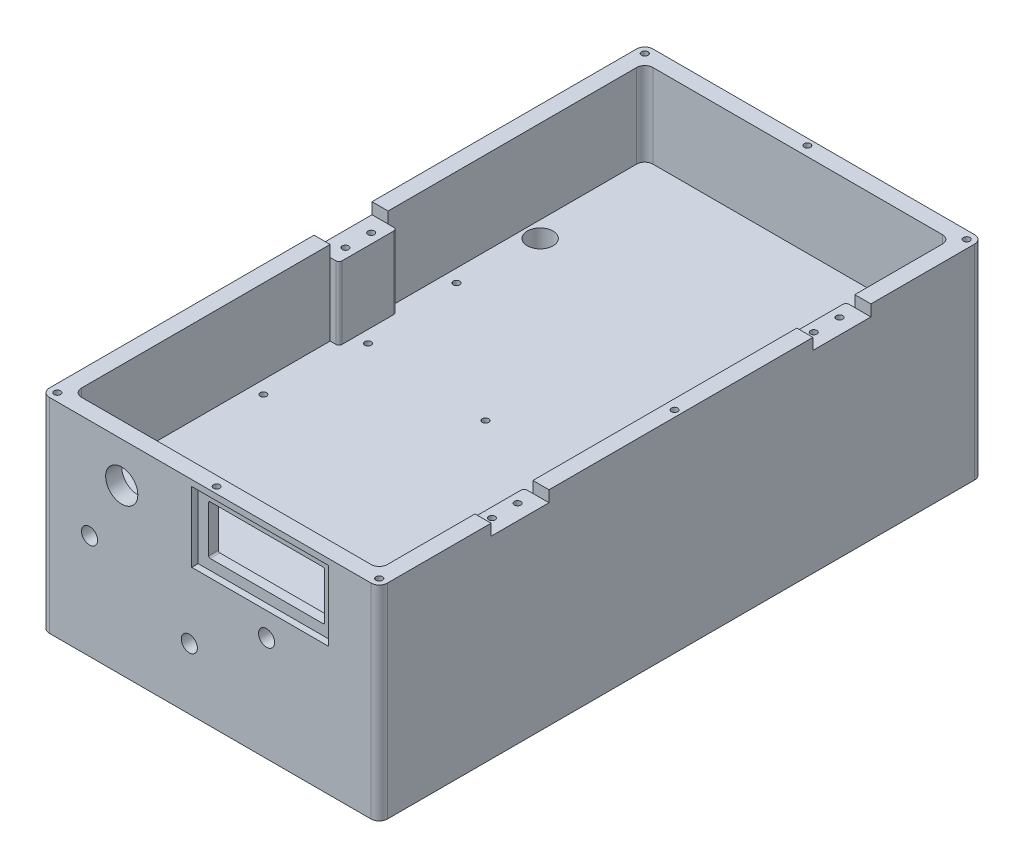
from build123d import *

# Parameters (mm, degrees)
SKETCH1_W           = 200
SKETCH1_H           = 400
BOSS_EXTRUDE1_DEPTH = 25
SKETCH2_R           = 1
SKETCH2_R_2         = 1.5
CUT_EXTRUDE1_DEPTH  = 5
BOSS_EXTRUDE2_DEPTH = 12
SKETCH10_R          = 2
CUT_EXTRUDE2_DEPTH  = 5
SKETCH11_R          = 2
CUT_EXTRUDE3_DEPTH  = 5
CUT_EXTRUDE4_DEPTH  = 157
SKETCH14_R          = 2
CUT_EXTRUDE5_DEPTH  = 5
SKETCH15_R          = 3.5
CUT_EXTRUDE6_DEPTH  = 175
SKETCH16_R          = 3.5
CUT_EXTRUDE7_DEPTH  = 20
SKETCH17_R          = 3.5
CUT_EXTRUDE8_DEPTH  = 270
SKETCH18_R          = 4
CUT_EXTRUDE9_DEPTH  = 7
SKETCH19_R          = 2
CUT_EXTRUDE10_DEPTH = 5
SKETCH20_W          = 200
SKETCH20_H          = 35
CUT_EXTRUDE11_DEPTH = 98
SKETCH21_R          = 1
CUT_EXTRUDE12_DEPTH = 5
BOSS_EXTRUDE3_START = 10
SKETCH27_W          = 200
SKETCH27_H          = 75
SKETCH27_R          = 3.5
BOSS_EXTRUDE3_DEPTH = 10
SKETCH28_R          = 5
CUT_EXTRUDE16_DEPTH = 10
SKETCH29_R          = 1.5
CUT_EXTRUDE17_DEPTH = 5
SKETCH30_W          = 375
SKETCH30_H          = 75
BOSS_EXTRUDE4_DEPTH = 10
SKETCH31_W          = 210
SKETCH31_H          = 75
BOSS_EXTRUDE5_DEPTH = 10
SKETCH32_W          = 375
SKETCH32_H          = 75
BOSS_EXTRUDE6_DEPTH = 10
SKETCH33_R          = 1.5
CUT_EXTRUDE18_DEPTH = 5
SKETCH34_W          = 210
SKETCH34_H          = 375
SKETCH34_W_2        = 190
SKETCH34_H_2        = 355
BOSS_EXTRUDE7_DEPTH = 52
SKETCH35_W          = 80
SKETCH35_H          = 30
CUT_EXTRUDE19_DEPTH = 35
SKETCH36_W          = 2
SKETCH36_H          = 357
CUT_EXTRUDE20_DEPTH = 1.5
SKETCH37_W          = 196
SKETCH37_H          = 2
CUT_EXTRUDE21_DEPTH = 1.5
SKETCH38_R          = 2
CUT_EXTRUDE22_DEPTH = 5
FILLET1_R           = 5
FILLET4_R           = 5
FILLET5_R           = 5
FILLET6_R           = 5
SKETCH41_R          = 5
CUT_EXTRUDE23_DEPTH = 28
SKETCH42_R          = 2
CUT_EXTRUDE24_DEPTH = 5
SKETCH43_R          = 2
CUT_EXTRUDE25_DEPTH = 5
SKETCH44_R          = 8
CUT_EXTRUDE26_DEPTH = 59
SKETCH45_R          = 2
CUT_EXTRUDE27_DEPTH = 5
SKETCH46_R          = 10
CUT_EXTRUDE28_DEPTH = 42
SKETCH47_R          = 5
CUT_EXTRUDE29_DEPTH = 20
BOSS_EXTRUDE8_DEPTH = 52
SKETCH51_W          = 15.5
SKETCH51_H          = 36
CUT_EXTRUDE31_DEPTH = 7
SKETCH52_R          = 2
CUT_EXTRUDE32_DEPTH = 5
FILLET7_R           = 2
CUT_EXTRUDE33_START = -5
SKETCH53_R          = 2
CUT_EXTRUDE33_DEPTH = 5
SKETCH56_R          = 1.5
CUT_EXTRUDE35_DEPTH = 5
MOVE_FACE1_BY       = 5
MOVE_FACE2_BY       = 3
MOVE_FACE3_BY       = 3.75
MOVE_FACE4_BY       = 3.25
SKETCH57_W          = 85
SKETCH57_H          = 43.5
CUT_EXTRUDE36_DEPTH = 4
FILLET8_R           = 1


with BuildPart() as part:
    # Sketch1 → Boss-Extrude1 (new body)
    with BuildSketch(Plane(origin=(0, 0, 0), x_dir=(1, 0, 0), z_dir=(0, 1, 0))):
        with Locations((100, 200)):
            Rectangle(SKETCH1_W, SKETCH1_H)
    extrude(amount=BOSS_EXTRUDE1_DEPTH)

    # Sketch2 → Cut-Extrude1 (cut)
    with BuildSketch(Plane.XZ):
        with Locations(Location((70, -320, 0), (0, 0, 270))):
            Circle(SKETCH2_R)
        with Locations(Location((68.3, -276.5, 0), (0, 0, 270))):
            Circle(SKETCH2_R)
        with Locations(Location((66, -139.3, 0), (0, 0, 270))):
            Circle(SKETCH2_R)
        with Locations(Location((50, -320, 0), (0, 0, 270))):
            Circle(SKETCH2_R)
        with Locations(Location((50, -300, 0), (0, 0, 270))):
            Circle(SKETCH2_R)
        with Locations(Location((70, -300, 0), (0, 0, 270))):
            Circle(SKETCH2_R)
        with Locations(Location((48.3, -276.5, 0), (0, 0, 270))):
            Circle(SKETCH2_R)
        with Locations(Location((46, -139.3, 0), (0, 0, 270))):
            Circle(SKETCH2_R)
        with Locations(Location((48.3, -256.5, 0), (0, 0, 270))):
            Circle(SKETCH2_R)
        with Locations(Location((46, -119.3, 0), (0, 0, 270))):
            Circle(SKETCH2_R)
        with Locations(Location((68.3, -256.5, 0), (0, 0, 270))):
            Circle(SKETCH2_R)
        with Locations(Location((66, -119.3, 0), (0, 0, 270))):
            Circle(SKETCH2_R)
        with Locations(Location((49.8, -220.8, 0), (0, 0, 270))):
            Circle(SKETCH2_R_2)
        with Locations(Location((65.606139731, -192.976162256, 0), (0, 0, 270))):
            Circle(SKETCH2_R_2)
        with Locations(Location((37.782301987, -177.170022525, 0), (0, 0, 270))):
            Circle(SKETCH2_R_2)
        with Locations(Location((21.976162256, -204.993860269, 0), (0, 0, 270))):
            Circle(SKETCH2_R_2)
        with Locations(Location((51.694220859, -185.07309239, 0), (0, 0, 270))):
            Circle(SKETCH2_R_2)
        with Locations(Location((8.064243384, -197.090790404, 0), (0, 0, 270))):
            Circle(SKETCH2_R_2)
    extrude(amount=-CUT_EXTRUDE1_DEPTH, mode=Mode.SUBTRACT)

    # Sketch9 → Boss-Extrude2 (add)
    with BuildSketch(Plane.XZ):
        Polygon((75, -330), (90, -330), (90, -315), (200, -315), (200, -400), (75, -400), (40, -400), (40, -330), align=None)
        Polygon((50, -99), (200, -99), (200, 0), (110, 0), (110, -79), (100, -79), (50, -79), align=None)
    extrude(amount=BOSS_EXTRUDE2_DEPTH)

    # Sketch10 → Cut-Extrude2 (cut)
    with BuildSketch(Plane.XZ.offset(12)):
        with Locations((82, -56.5)):
            Circle(SKETCH10_R)
        with Locations(Location((119, -56.5, 0), (0, 0, 270))):
            Circle(SKETCH10_R)
        with Locations(Location((59.7, -86.5, 0), (0, 0, 270))):
            Circle(SKETCH10_R)
        with Locations(Location((99, -90, 0), (0, 0, 270))):
            Circle(SKETCH10_R)
        with Locations(Location((138.2, -321.7, 0), (0, 0, 270))):
            Circle(SKETCH10_R)
        with Locations(Location((119.5, -370, 0), (0, 0, 270))):
            Circle(SKETCH10_R)
        with Locations(Location((101.2, -321.7, 0), (0, 0, 270))):
            Circle(SKETCH10_R)
        with Locations(Location((82, -370, 0), (0, 0, 270))):
            Circle(SKETCH10_R)
    extrude(amount=-CUT_EXTRUDE2_DEPTH, mode=Mode.SUBTRACT)

    # Sketch11 → Cut-Extrude3 (cut)
    with BuildSketch(Plane(origin=(0, 25, 0), x_dir=(1, 0, 0), z_dir=(0, 1, 0))):
        with Locations(Location((161, 200, 0), (0, 0, 270))):
            Circle(SKETCH11_R)
        with Locations(Location((91, 200, 0), (0, 0, 270))):
            Circle(SKETCH11_R)
        with Locations(Location((91, 42, 0), (0, 0, 270))):
            Circle(SKETCH11_R)
        with Locations(Location((161, 42, 0), (0, 0, 270))):
            Circle(SKETCH11_R)
    extrude(amount=-CUT_EXTRUDE3_DEPTH, mode=Mode.SUBTRACT)

    # Sketch13 → Cut-Extrude4 (cut)
    with BuildSketch(Plane.XZ):
        Polygon((165.75, -235), (144.75, -235), (144.75, -266), (155.25, -266), (165.75, -266), align=None)
    extrude(amount=-CUT_EXTRUDE4_DEPTH, mode=Mode.SUBTRACT)

    # Sketch14 → Cut-Extrude5 (cut)
    with BuildSketch(Plane.XZ.offset(12)):
        with Locations(Location((165.411124446, -340.161124446, 0), (0, 0, 270))):
            Circle(SKETCH14_R)
        with Locations(Location((49.838875554, -340.161124446, 0), (0, 0, 270))):
            Circle(SKETCH14_R)
    extrude(amount=-CUT_EXTRUDE5_DEPTH, mode=Mode.SUBTRACT)

    # Sketch15 → Cut-Extrude6 (cut)
    with BuildSketch(Plane.XY):
        with Locations((130, 15)):
            Circle(SKETCH15_R)
    extrude(amount=-CUT_EXTRUDE6_DEPTH, mode=Mode.SUBTRACT)

    # Sketch16 → Cut-Extrude7 (cut)
    with BuildSketch(Plane.XZ):
        with Locations(Location((130, -170, 0), (0, 0, 270))):
            Circle(SKETCH16_R)
        with Locations(Location((20, -265, 0), (0, 0, 270))):
            Circle(SKETCH16_R)
    extrude(amount=-CUT_EXTRUDE7_DEPTH, mode=Mode.SUBTRACT)

    # Sketch17 → Cut-Extrude8 (cut)
    with BuildSketch(Plane.XY):
        with Locations((20, 15)):
            Circle(SKETCH17_R)
    extrude(amount=-CUT_EXTRUDE8_DEPTH, mode=Mode.SUBTRACT)

    # Sketch18 → Cut-Extrude9 (cut)
    with BuildSketch(Plane.XZ):
        with Locations(Location((130, -170, 0), (0, 0, 270))):
            Circle(SKETCH18_R)
        with Locations(Location((20, -265, 0), (0, 0, 270))):
            Circle(SKETCH18_R)
    extrude(amount=-CUT_EXTRUDE9_DEPTH, mode=Mode.SUBTRACT)

    # Sketch19 → Cut-Extrude10 (cut)
    with BuildSketch(Plane.XZ):
        with Locations(Location((181.25, -250.5, 0), (0, 0, 270))):
            Circle(SKETCH19_R)
        with Locations(Location((131.25, -250.5, 0), (0, 0, 270))):
            Circle(SKETCH19_R)
    extrude(amount=-CUT_EXTRUDE10_DEPTH, mode=Mode.SUBTRACT)

    # Sketch20 → Cut-Extrude11 (cut)
    with BuildSketch(Plane.XZ.offset(12)):
        with Locations((100, -17.5)):
            Rectangle(SKETCH20_W, SKETCH20_H)
    extrude(amount=-CUT_EXTRUDE11_DEPTH, mode=Mode.SUBTRACT)

    # Sketch21 → Cut-Extrude12 (cut)
    with BuildSketch(Plane.XZ):
        with Locations(Location((72, -46.5, 0), (0, 0, 270))):
            Circle(SKETCH21_R)
        with Locations(Location((92, -46.5, 0), (0, 0, 270))):
            Circle(SKETCH21_R)
        with Locations(Location((92, -66.5, 0), (0, 0, 270))):
            Circle(SKETCH21_R)
        with Locations(Location((72, -66.5, 0), (0, 0, 270))):
            Circle(SKETCH21_R)
    extrude(amount=-CUT_EXTRUDE12_DEPTH, mode=Mode.SUBTRACT)

    # Sketch27 → Boss-Extrude3 (add)
    with BuildSketch(Plane.XY.offset(-35).offset(BOSS_EXTRUDE3_START)):
        with Locations((100, -12.5)):
            Rectangle(SKETCH27_W, SKETCH27_H)
        with Locations((130, 15)):
            Circle(SKETCH27_R, mode=Mode.SUBTRACT)
        with Locations((20, 15)):
            Circle(SKETCH27_R, mode=Mode.SUBTRACT)
    extrude(amount=-BOSS_EXTRUDE3_DEPTH)

    # Sketch28 → Cut-Extrude16 (cut)
    with BuildSketch(Plane.XY.offset(-25)):
        with Locations((82, -12)):
            Circle(SKETCH28_R)
    extrude(amount=-CUT_EXTRUDE16_DEPTH, mode=Mode.SUBTRACT)

    # Sketch29 → Cut-Extrude17 (cut)
    with BuildSketch(Plane.XZ):
        with Locations(Location((103, -59.5, 0), (0, 0, 270))):
            Circle(SKETCH29_R)
        with Locations(Location((103, -63.5, 0), (0, 0, 270))):
            Circle(SKETCH29_R)
    extrude(amount=-CUT_EXTRUDE17_DEPTH, mode=Mode.SUBTRACT)

    # Sketch30 → Boss-Extrude4 (add)
    with BuildSketch(Plane.ZY):
        with Locations((-212.5, -12.5)):
            Rectangle(SKETCH30_W, SKETCH30_H)
    extrude(amount=BOSS_EXTRUDE4_DEPTH)

    # Sketch31 → Boss-Extrude5 (add)
    with BuildSketch(Plane(origin=(0, 0, -400), x_dir=(-1, 0, 0), z_dir=(0, 0, -1))):
        with Locations((-95, -12.5)):
            Rectangle(SKETCH31_W, SKETCH31_H)
    extrude(amount=-BOSS_EXTRUDE5_DEPTH)

    # Sketch32 → Boss-Extrude6 (add)
    with BuildSketch(Plane(origin=(200, 0, 0), x_dir=(0, 0, -1), z_dir=(1, 0, 0))):
        with Locations((212.5, -12.5)):
            Rectangle(SKETCH32_W, SKETCH32_H)
    extrude(amount=-BOSS_EXTRUDE6_DEPTH)

    # Sketch33 → Cut-Extrude18 (cut)
    with BuildSketch(Plane.XZ.offset(12)):
        with Locations(Location((95, -341, 0), (0, 0, 270))):
            Circle(SKETCH33_R)
        with Locations(Location((140, -341, 0), (0, 0, 270))):
            Circle(SKETCH33_R)
    extrude(amount=-CUT_EXTRUDE18_DEPTH, mode=Mode.SUBTRACT)

    # Sketch34 → Boss-Extrude7 (add)
    with BuildSketch(Plane(origin=(0, 25, 0), x_dir=(1, 0, 0), z_dir=(0, 1, 0))):
        with Locations((95, 212.5)):
            Rectangle(SKETCH34_W, SKETCH34_H)
        with Locations((95, 212.5)):
            Rectangle(SKETCH34_W_2, SKETCH34_H_2, mode=Mode.SUBTRACT)
    extrude(amount=BOSS_EXTRUDE7_DEPTH)

    # Sketch35 → Cut-Extrude19 (cut)
    with BuildSketch(Plane.XY.offset(-25)):
        with Locations((127, 55)):
            Rectangle(SKETCH35_W, SKETCH35_H)
    extrude(amount=-CUT_EXTRUDE19_DEPTH, mode=Mode.SUBTRACT)

    # Sketch36 → Cut-Extrude20 (cut)
    with BuildSketch(Plane.XZ.offset(50)):
        with Locations((-2, -212.5)):
            Rectangle(SKETCH36_W, SKETCH36_H)
        with Locations((192, -212.5)):
            Rectangle(SKETCH36_W, SKETCH36_H)
    extrude(amount=-CUT_EXTRUDE20_DEPTH, mode=Mode.SUBTRACT)

    # Sketch37 → Cut-Extrude21 (cut)
    with BuildSketch(Plane.XZ.offset(50)):
        with Locations((95, -392)):
            Rectangle(SKETCH37_W, SKETCH37_H)
        with Locations((95, -33)):
            Rectangle(SKETCH37_W, SKETCH37_H)
    extrude(amount=-CUT_EXTRUDE21_DEPTH, mode=Mode.SUBTRACT)

    # Sketch38 → Cut-Extrude22 (cut)
    with BuildSketch(Plane.XZ.offset(50)):
        with Locations(Location((195, -30, 0), (0, 0, 270))):
            Circle(SKETCH38_R)
        with Locations(Location((95, -396, 0), (0, 0, 270))):
            Circle(SKETCH38_R)
        with Locations(Location((95, -29, 0), (0, 0, 270))):
            Circle(SKETCH38_R)
        with Locations(Location((-6, -212.5, 0), (0, 0, 270))):
            Circle(SKETCH38_R)
        with Locations(Location((196, -212.5, 0), (0, 0, 270))):
            Circle(SKETCH38_R)
        with Locations(Location((-5, -30, 0), (0, 0, 270))):
            Circle(SKETCH38_R)
        with Locations(Location((-5, -395, 0), (0, 0, 270))):
            Circle(SKETCH38_R)
        with Locations(Location((195, -395, 0), (0, 0, 270))):
            Circle(SKETCH38_R)
    extrude(amount=-CUT_EXTRUDE22_DEPTH, mode=Mode.SUBTRACT)

    # Fillet1
    fillet1_edges = [part.edges().sort_by_distance(p)[0] for p in [
        (200, 13.5, -25),
        (-10, 13.5, -25),
        (-10, 13.5, -400),
        (200, 13.5, -400),
    ]]
    fillet(fillet1_edges, radius=FILLET1_R)

    # Fillet4
    fillet4_edges = [part.edges().sort_by_distance(p)[0] for p in [
        (0, -25, -35),
        (0, -25, -390),
        (190, -31, -390),
        (190, -31, -35),
    ]]
    fillet(fillet4_edges, radius=FILLET4_R)

    # Fillet5
    fillet5_edges = [part.edges().sort_by_distance(p)[0] for p in [
        (-1, -49.25, -34),
        (-1, -49.25, -391),
        (191, -49.25, -391),
        (191, -49.25, -34),
        (-3, -49.25, -393),
        (193, -49.25, -393),
        (-3, -49.25, -32),
        (193, -49.25, -32),
    ]]
    fillet(fillet5_edges, radius=FILLET5_R)

    # Fillet6
    fillet6_edges = [part.edges().sort_by_distance(p)[0] for p in [
        (190, 51, -35),
        (190, 51, -390),
        (0, 51, -390),
        (0, 51, -35),
    ]]
    fillet(fillet6_edges, radius=FILLET6_R)

    # Sketch41 → Cut-Extrude23 (cut)
    with BuildSketch(Plane(origin=(0, 0, -400), x_dir=(-1, 0, 0), z_dir=(0, 0, -1))):
        with Locations((-119.5, -24.7)):
            Circle(SKETCH41_R)
    extrude(amount=-CUT_EXTRUDE23_DEPTH, mode=Mode.SUBTRACT)

    # Sketch42 → Cut-Extrude24 (cut)
    with BuildSketch(Plane.XZ.offset(12)):
        with Locations(Location((155, -375, 0), (0, 0, 270))):
            Circle(SKETCH42_R)
    extrude(amount=-CUT_EXTRUDE24_DEPTH, mode=Mode.SUBTRACT)

    # Sketch43 → Cut-Extrude25 (cut)
    with BuildSketch(Plane.XZ):
        with Locations(Location((10, -385, 0), (0, 0, 270))):
            Circle(SKETCH43_R)
        with Locations(Location((10, -364, 0), (0, 0, 270))):
            Circle(SKETCH43_R)
    extrude(amount=-CUT_EXTRUDE25_DEPTH, mode=Mode.SUBTRACT)

    # Sketch44 → Cut-Extrude26 (cut)
    with BuildSketch(Plane.XZ):
        with Locations(Location((10, -315, 0), (0, 0, 270))):
            Circle(SKETCH44_R)
    extrude(amount=-CUT_EXTRUDE26_DEPTH, mode=Mode.SUBTRACT)

    # Sketch45 → Cut-Extrude27 (cut)
    with BuildSketch(Plane(origin=(0, 25, 0), x_dir=(1, 0, 0), z_dir=(0, 1, 0))):
        with Locations(Location((8, 265, 0), (0, 0, 270))):
            Circle(SKETCH45_R)
        with Locations(Location((8, 145, 0), (0, 0, 270))):
            Circle(SKETCH45_R)
        with Locations(Location((8, 85, 0), (0, 0, 270))):
            Circle(SKETCH45_R)
        with Locations(Location((13, 205, 0), (0, 0, 270))):
            Circle(SKETCH45_R)
    extrude(amount=-CUT_EXTRUDE27_DEPTH, mode=Mode.SUBTRACT)

    # Sketch46 → Cut-Extrude28 (cut)
    with BuildSketch(Plane.XY.offset(-25)):
        with Locations((40, 52)):
            Circle(SKETCH46_R)
    extrude(amount=-CUT_EXTRUDE28_DEPTH, mode=Mode.SUBTRACT)

    # Sketch47 → Cut-Extrude29 (cut)
    with BuildSketch(Plane.XY.offset(-25)):
        with Locations((20, 15)):
            Circle(SKETCH47_R)
        with Locations((130, 15)):
            Circle(SKETCH47_R)
    extrude(amount=-CUT_EXTRUDE29_DEPTH, mode=Mode.SUBTRACT)

    # Sketch49 → Boss-Extrude8 (add)
    with BuildSketch(Plane(origin=(0, 77, 0), x_dir=(1, 0, 0), z_dir=(0, 1, 0))):
        Polygon((0, 212.5), (0, 230.5), (5.5, 230.5), (5.5, 194.5), (0, 194.5), align=None)
        Polygon((190, 312.5), (190, 330.5), (184.5, 330.5), (184.5, 294.5), (190, 294.5), align=None)
        Polygon((190, 130.5), (190, 112.5), (190, 94.5), (184.5, 94.5), (184.5, 130.5), align=None)
    extrude(amount=-BOSS_EXTRUDE8_DEPTH)

    # Sketch51 → Cut-Extrude31 (cut)
    with BuildSketch(Plane(origin=(0, 77, 0), x_dir=(1, 0, 0), z_dir=(0, 1, 0))):
        with Locations((192.25, 312.5)):
            Rectangle(SKETCH51_W, SKETCH51_H)
        with Locations((192.25, 112.5)):
            Rectangle(SKETCH51_W, SKETCH51_H)
        with Locations((-2.25, 212.5)):
            Rectangle(SKETCH51_W, SKETCH51_H)
    extrude(amount=-CUT_EXTRUDE31_DEPTH, mode=Mode.SUBTRACT)

    # Sketch52 → Cut-Extrude32 (cut)
    with BuildSketch(Plane(origin=(0, 70, 0), x_dir=(1, 0, 0), z_dir=(0, 1, 0))):
        with Locations(Location((-0.5, 220.5, 0), (0, 0, 270))):
            Circle(SKETCH52_R)
        with Locations(Location((-0.5, 204.5, 0), (0, 0, 270))):
            Circle(SKETCH52_R)
        with Locations(Location((190.5, 104.5, 0), (0, 0, 270))):
            Circle(SKETCH52_R)
        with Locations(Location((190.5, 120.5, 0), (0, 0, 270))):
            Circle(SKETCH52_R)
        with Locations(Location((190.5, 320.5, 0), (0, 0, 270))):
            Circle(SKETCH52_R)
        with Locations(Location((190.5, 304.5, 0), (0, 0, 270))):
            Circle(SKETCH52_R)
    extrude(amount=-CUT_EXTRUDE32_DEPTH, mode=Mode.SUBTRACT)

    # Fillet7
    fillet7_edges = [part.edges().sort_by_distance(p)[0] for p in [
        (5.5, 47.5, -230.5),
        (5.5, 47.5, -194.5),
        (184.5, 47.5, -294.5),
        (184.5, 47.5, -330.5),
        (184.5, 47.5, -130.5),
        (184.5, 47.5, -94.5),
    ]]
    fillet(fillet7_edges, radius=FILLET7_R)

    # Sketch53 → Cut-Extrude33 (cut)
    with BuildSketch(Plane(origin=(0, 77, 0), x_dir=(1, 0, 0), z_dir=(0, 1, 0)).offset(CUT_EXTRUDE33_START)):
        with Locations(Location((-5, 30, 0), (0, 0, 90))):
            Circle(SKETCH53_R)
        with Locations(Location((95, 29, 0), (0, 0, 90))):
            Circle(SKETCH53_R)
        with Locations(Location((195, 30, 0), (0, 0, 90))):
            Circle(SKETCH53_R)
        with Locations(Location((196, 212.5, 0), (0, 0, 90))):
            Circle(SKETCH53_R)
        with Locations(Location((195, 395, 0), (0, 0, 90))):
            Circle(SKETCH53_R)
        with Locations(Location((95, 396, 0), (0, 0, 90))):
            Circle(SKETCH53_R)
        with Locations(Location((-5, 395, 0), (0, 0, 90))):
            Circle(SKETCH53_R)
    extrude(amount=CUT_EXTRUDE33_DEPTH, mode=Mode.SUBTRACT)

    # Sketch56 → Cut-Extrude35 (cut)
    with BuildSketch(Plane.XZ):
        with Locations(Location((161.25, -231.5, 0), (0, 0, 270))):
            Circle(SKETCH56_R)
        with Locations(Location((149.25, -231.5, 0), (0, 0, 270))):
            Circle(SKETCH56_R)
        with Locations(Location((161.25, -269.5, 0), (0, 0, 270))):
            Circle(SKETCH56_R)
        with Locations(Location((149.25, -269.5, 0), (0, 0, 270))):
            Circle(SKETCH56_R)
    extrude(amount=-CUT_EXTRUDE35_DEPTH, mode=Mode.SUBTRACT)

    # Move Face1: a face moved outward by 5.0
    extrude(part.faces().sort_by_distance((167, 55, -30))[0], amount=MOVE_FACE1_BY, dir=(-1, 0, 0))

    # Move Face2: a face moved outward by 3.0
    extrude(part.faces().sort_by_distance((87, 55, -30))[0], amount=MOVE_FACE2_BY, dir=(1, 0, 0))

    # Move Face3: a face moved inward by 3.75
    extrude(part.faces().sort_by_distance((126, 40, -30))[0], amount=MOVE_FACE3_BY, dir=(0, -1, 0), mode=Mode.SUBTRACT)

    # Move Face4: a face moved outward by 3.25
    extrude(part.faces().sort_by_distance((126, 70, -30))[0], amount=MOVE_FACE4_BY, dir=(0, -1, 0))

    # Sketch57 → Cut-Extrude36 (cut)
    with BuildSketch(Plane.XY.offset(-25)):
        with Locations((126, 51.5)):
            Rectangle(SKETCH57_W, SKETCH57_H)
    extrude(amount=-CUT_EXTRUDE36_DEPTH, mode=Mode.SUBTRACT)

    # Fillet8
    fillet8_edges = [part.edges().sort_by_distance(p)[0] for p in [
        (162, 66.75, -32),
        (162, 36.25, -32),
        (90, 36.25, -32),
        (90, 66.75, -32),
    ]]
    fillet(fillet8_edges, radius=FILLET8_R)


solid = part.part
